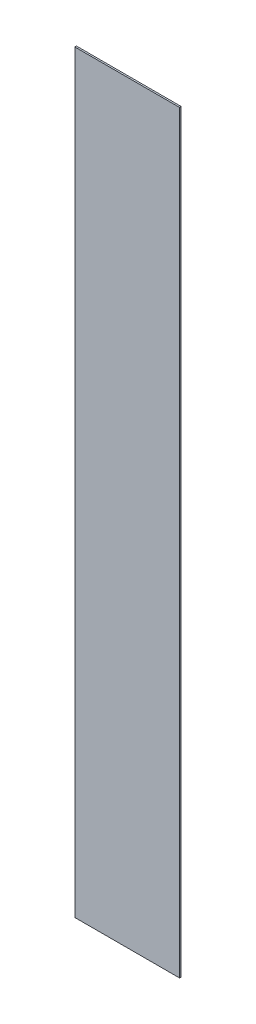
from build123d import *

# Parameters (mm, degrees)
SKETCH_1_W      = 321
SKETCH_1_H      = 2310
EXTRUDE_1_DEPTH = 5


with BuildPart() as part:
    # 草图1 → 凸台-拉伸1 (new body)
    with BuildSketch(Plane.XY):
        Rectangle(SKETCH_1_W, SKETCH_1_H)
    extrude(amount=EXTRUDE_1_DEPTH)


solid = part.part
